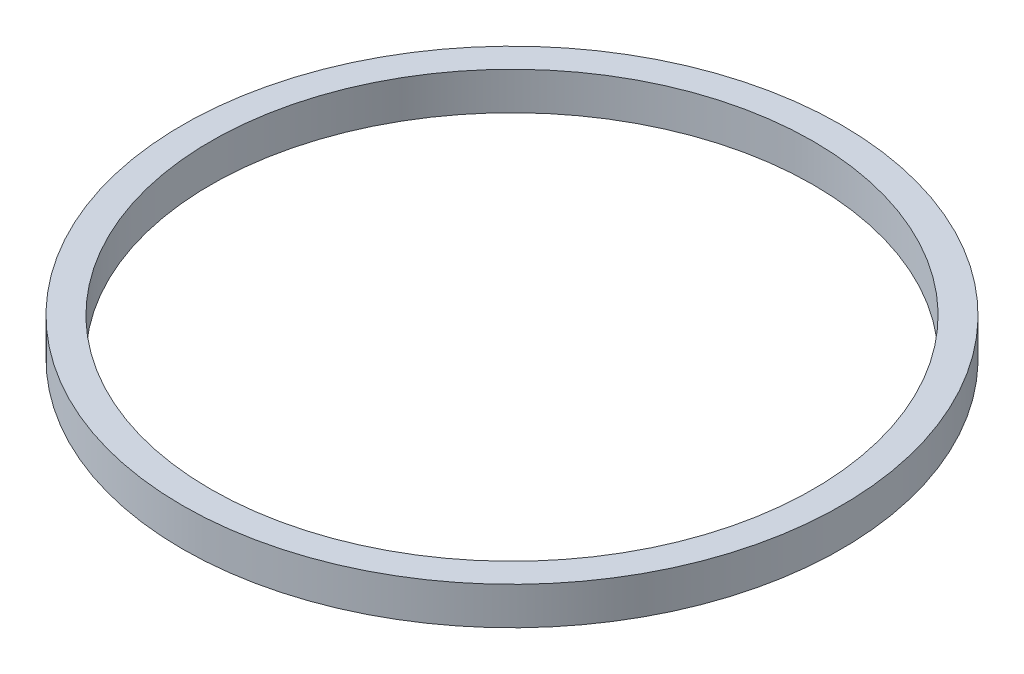
SolidWorks part; units mm, degrees
ref_plane "Front Plane" through (0, 0, 0) normal (0, 0, 1) x (1, 0, 0)
ref_plane "Top Plane" through (0, 0, 0) normal (0, 1, 0) x (1, 0, 0)
ref_plane "Right Plane" through (0, 0, 0) normal (1, 0, 0) x (0, 0, -1)
other "Configuration Table"
sketch "Sketch1" plane through (0, 0, 0) normal (0, 1, 0) x (1, 0, 0)
  circle A0 centre (0, 0) radius 17.5
  circle A1 centre (0, 0) radius 16
  dimension "D1" = 35
  dimension "D2" = 32
extrude "Boss-Extrude1" add sketch "Sketch1" along normal mid plane 2
